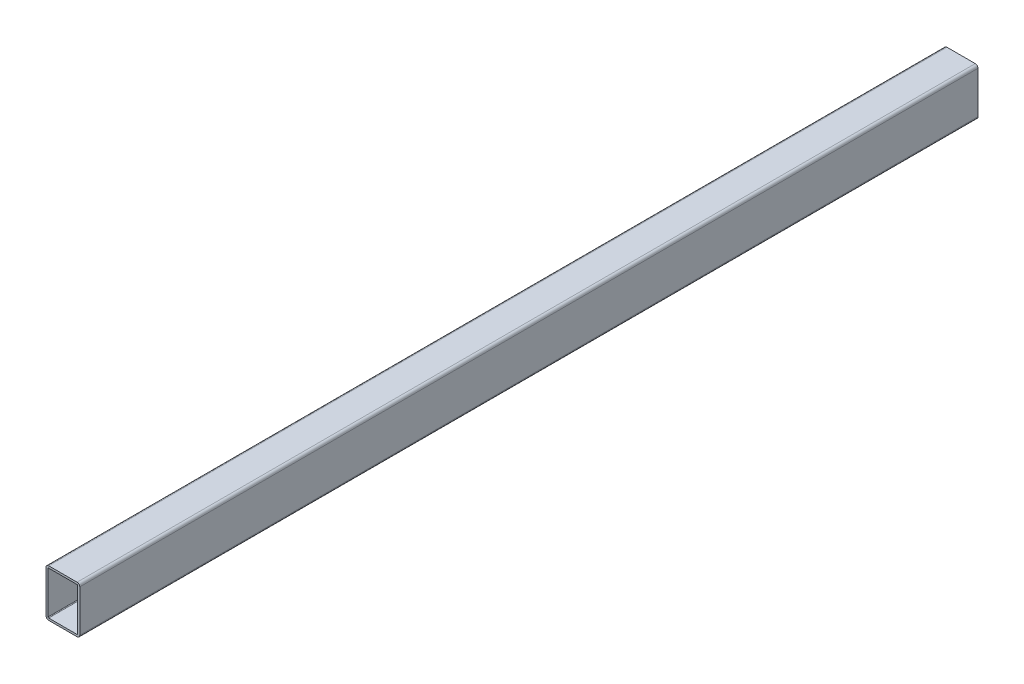
SolidWorks part; units mm, degrees
material "AISI 1045 钢，冷拔"
ref_plane "Front Plane" through (0, 0, 0) normal (0, 0, 1) x (1, 0, 0)
ref_plane "Top Plane" through (0, 0, 0) normal (0, 1, 0) x (1, 0, 0)
ref_plane "Right Plane" through (0, 0, 0) normal (1, 0, 0) x (0, 0, -1)
sketch "Sketch1" plane through (0, 0, 0) normal (0, 0, 1) x (1, 0, 0)
  line L1 (-21, -35) -> (21, -35)
  line L2 (-25, -31) -> (-25, 31)
  line L3 (-21, 35) -> (21, 35)
  line L4 (25, -31) -> (25, 31)
  line L5 (-25, -35) -> (25, 35) construction
  line L6 (-25, 35) -> (25, -35) construction
  arc A0 (-21, -35) -> (-25, -31) centre (-21, -31) cw
  arc A1 (21, -35) -> (25, -31) centre (21, -31) ccw
  arc A2 (21, 35) -> (25, 31) centre (21, 31) cw
  arc A3 (-25, 31) -> (-21, 35) centre (-21, 31) cw
  point P0 (0, 0)
  dimension "D3" = 4
  dimension "D1" = 50
  dimension "D2" = 70
extrude "Extrude-Thin1" add sketch "Sketch1" along normal blind 1330 thin thin type one direction reverse wall 3
